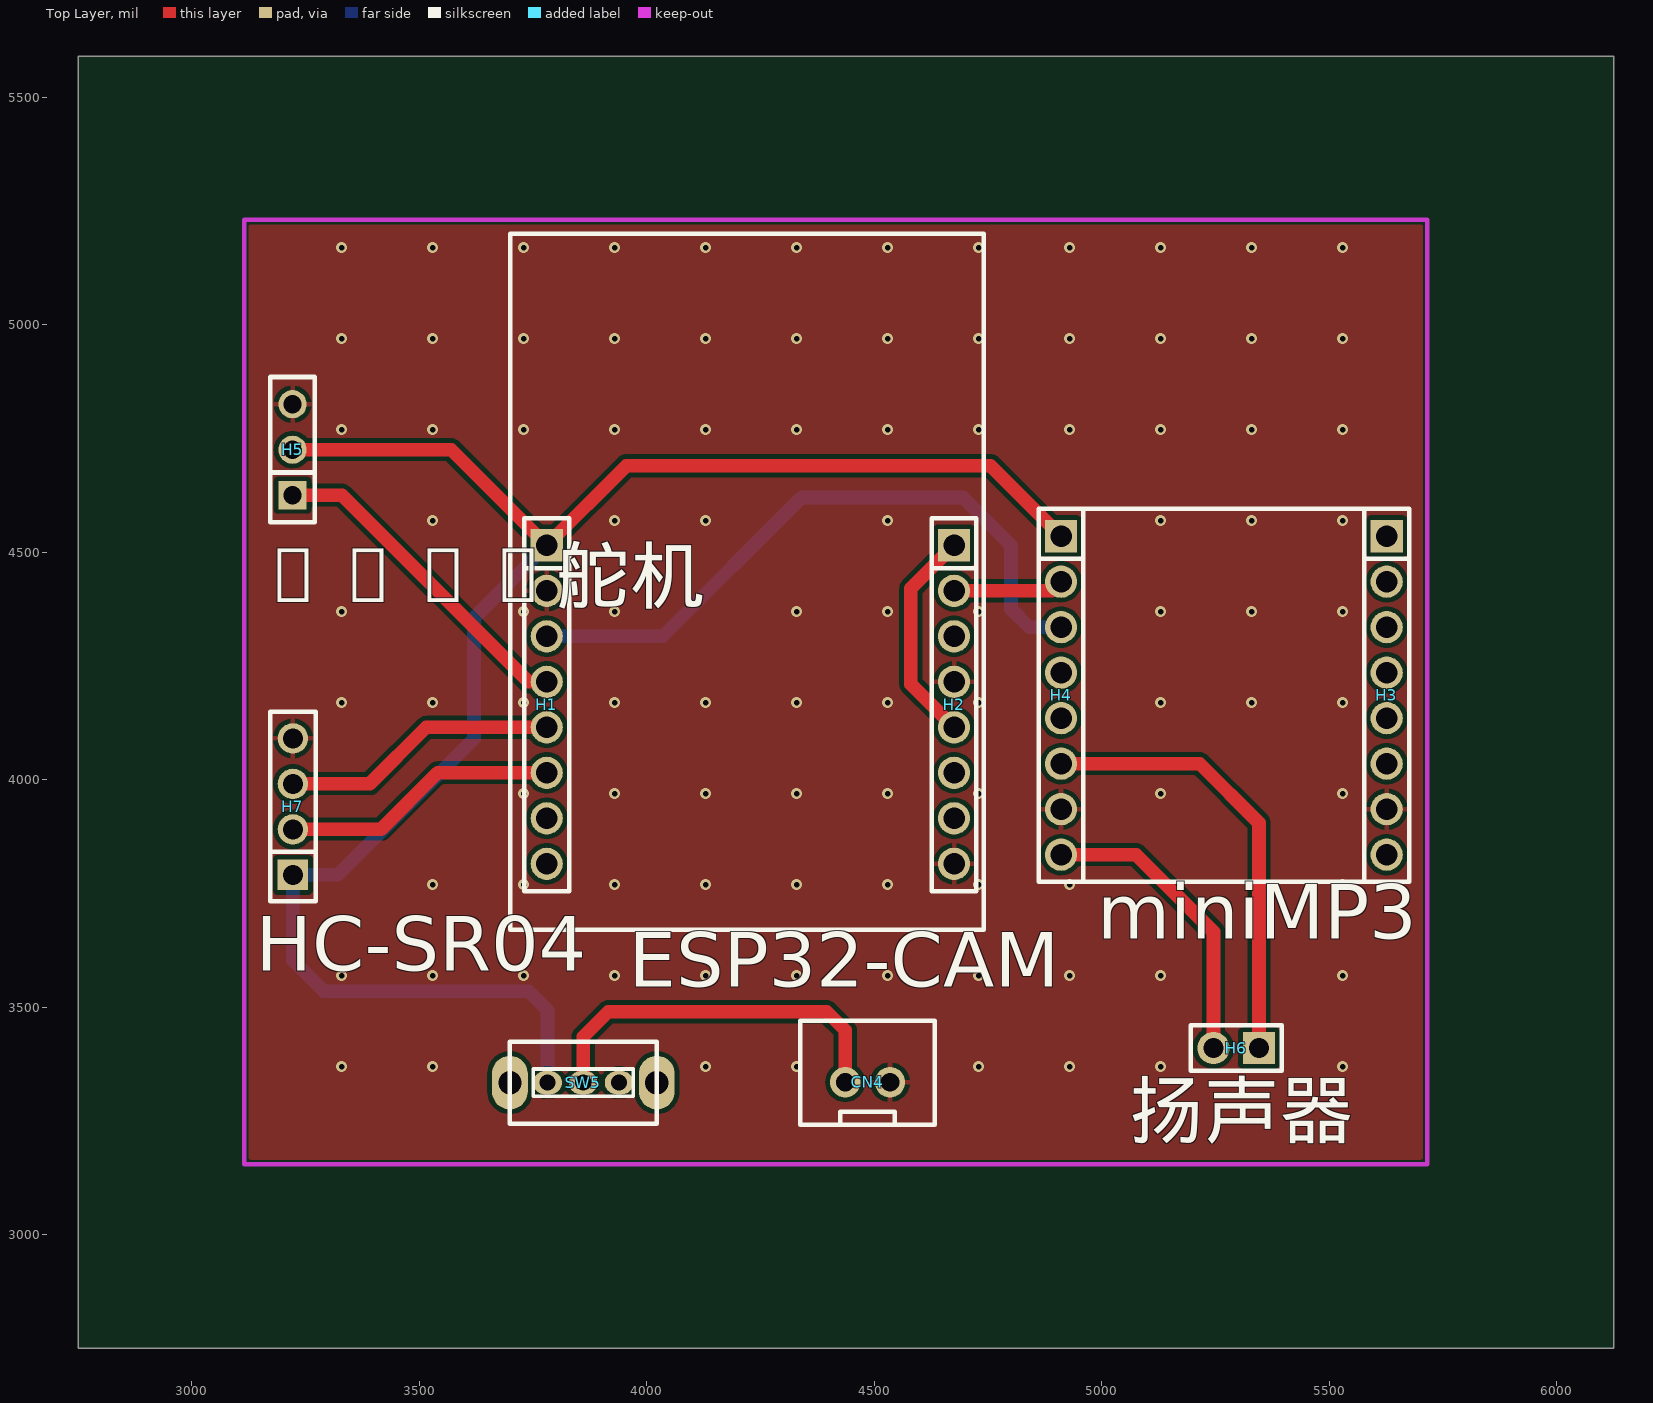
[diagram p0: Top Layer view]
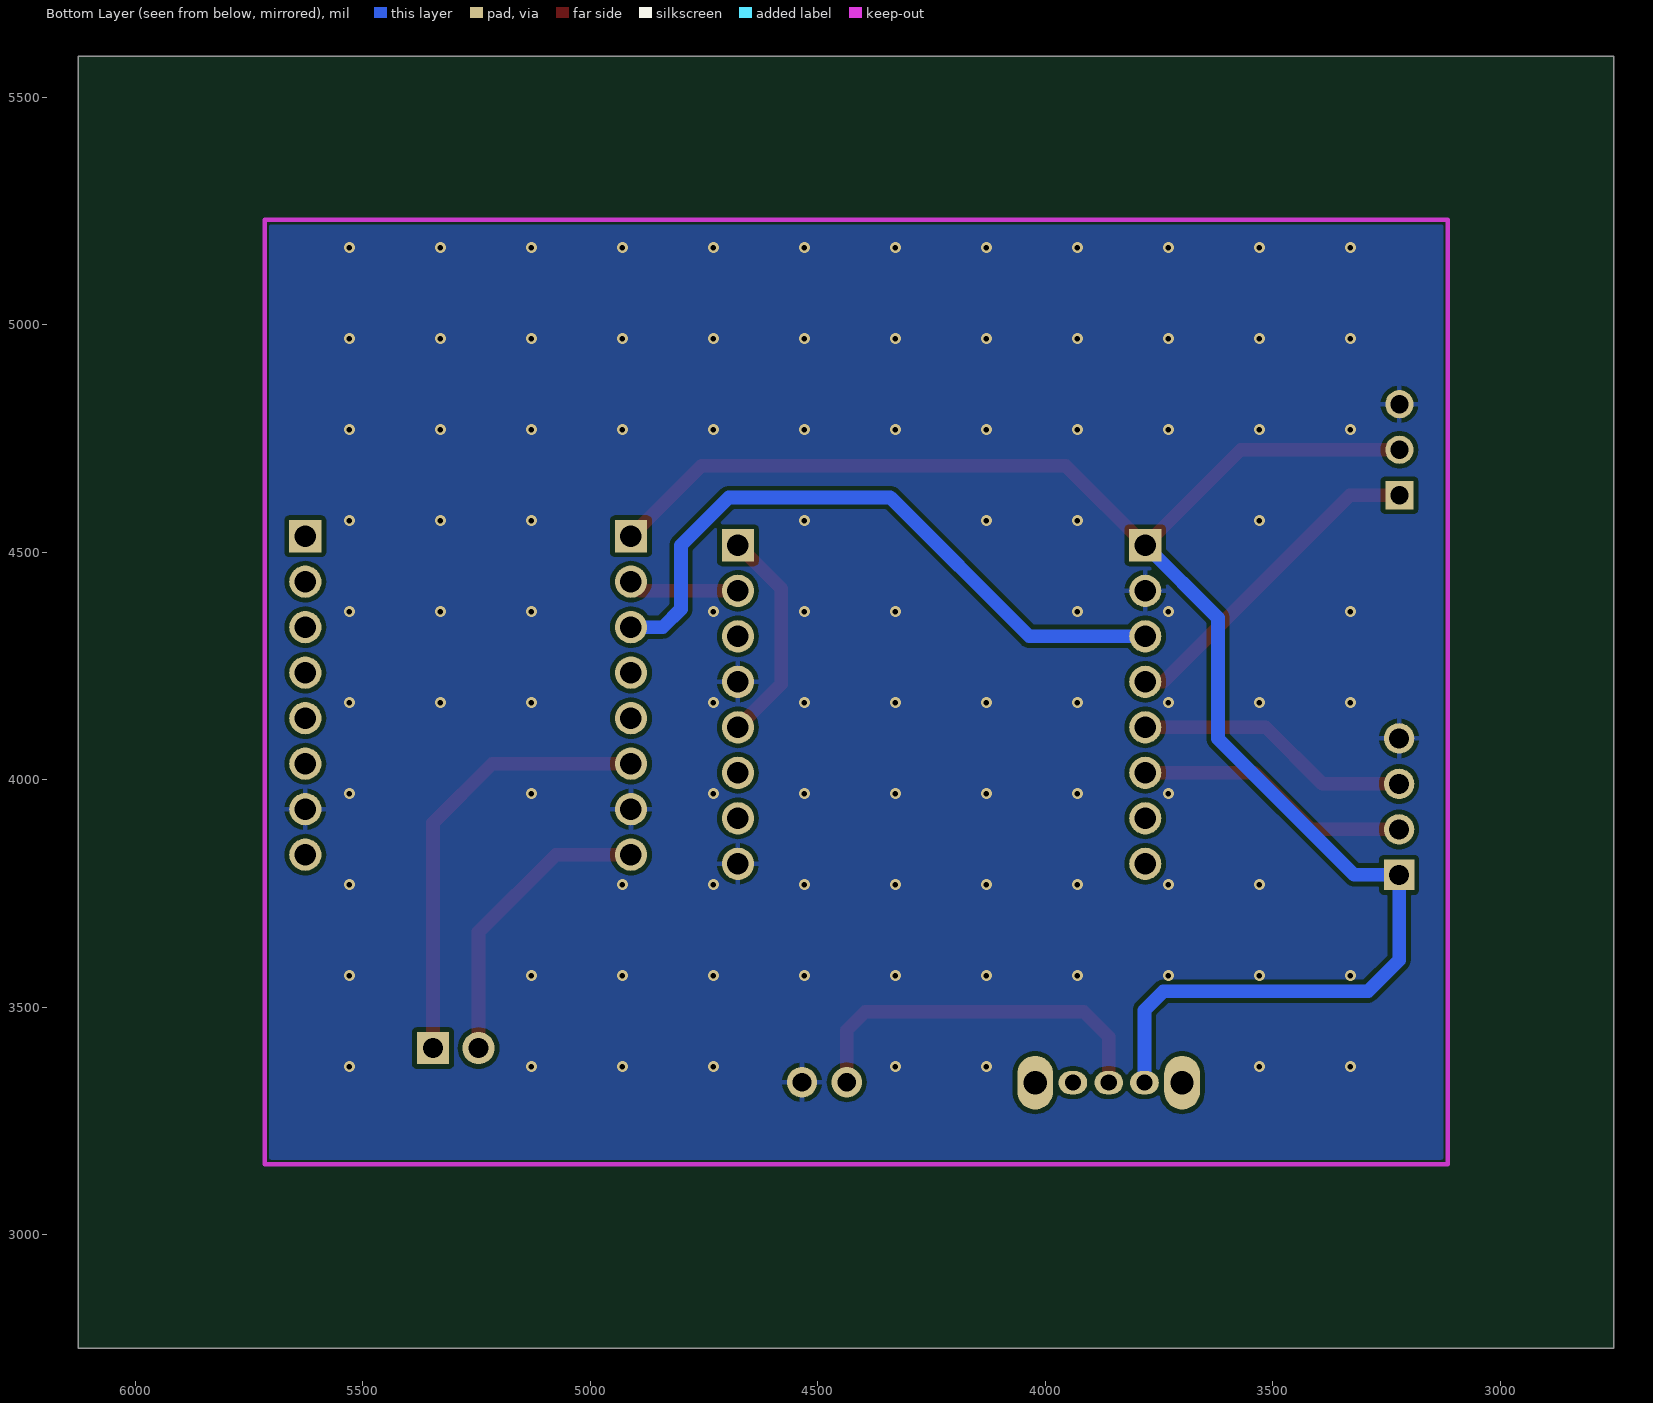
[diagram p1: Bottom Layer view, seen from below]
# Altium PCB MISC51682.pcbdoc
Units mil, origin at the board's own origin, x right, y up, seen from the top; angles counter-clockwise.
Board outline 3375 x 2840 mil, 2 copper layers (Top Layer, Bottom Layer), stack 62.206 mil thick; 9 components, 16 nets, 48 pads, 99 vias.

## Layer stack, top to bottom
Top Solder Mask Layer: solder mask 0.394, Dk 3.3
Top Layer: signal copper 1.379
Dielectric1: surface 59.449, FR4, Dk 4.5
Bottom Layer: signal copper 1.378
Bottom Solder Mask Layer: solder mask 0.394, Dk 3.3

## Board outline
6125,2750 2750,2750 2750,5590 6125,5590

## Design rules (kind name [scope] priority, off if disabled: settings)
BoardOutlineClearance copperThickness2oz_1 [All] p2 off: genericclearance=7.99 ignorepadtopadclearanceinfootprint=FALSE except(0: Arc-SplitContinuation Track-SplitContinuation SMDPad-SplitContinuation THPad-SplitContinuation Via-SplitContinuation Fill-SplitContinuation Region-SplitContinuation Poly-SplitContinuation Text-SplitContinuation Hole-SplitContinuation; 5.98: Arc-CutoutEdge Track-CutoutEdge SMDPad-CutoutEdge THPad-CutoutEdge Via-CutoutEdge Text-CutoutEdge; 6.9: Hole-OutlineEdge Hole-CutoutEdge; 10: Poly-OutlineEdge Poly-CutoutEdge; 11.81: Arc-OutlineEdge Track-OutlineEdge SMDPad-OutlineEdge THPad-OutlineEdge Via-OutlineEdge Fill-OutlineEdge Region-OutlineEdge Text-OutlineEdge Fill-CutoutEdge Region-CutoutEdge)
BoardOutlineClearance Plane_innerPlane_1 [All] p4 off: genericclearance=4.02 ignorepadtopadclearanceinfootprint=FALSE except(0: Arc-SplitContinuation Track-SplitContinuation SMDPad-SplitContinuation THPad-SplitContinuation Via-SplitContinuation Fill-SplitContinuation Region-SplitContinuation Poly-SplitContinuation Text-SplitContinuation Hole-SplitContinuation; 5.98: Arc-CutoutEdge Track-CutoutEdge SMDPad-CutoutEdge THPad-CutoutEdge Via-CutoutEdge Text-CutoutEdge; 6.9: Hole-OutlineEdge Hole-CutoutEdge; 10: Poly-OutlineEdge Poly-CutoutEdge; 11.81: Arc-OutlineEdge Track-OutlineEdge SMDPad-OutlineEdge THPad-OutlineEdge Via-OutlineEdge Fill-OutlineEdge Region-OutlineEdge Text-OutlineEdge Fill-CutoutEdge Region-CutoutEdge)
BoardOutlineClearance Copper_copperRegion_1 [All] p6 off: genericclearance=4.02 ignorepadtopadclearanceinfootprint=FALSE except(0: Arc-SplitContinuation Track-SplitContinuation SMDPad-SplitContinuation THPad-SplitContinuation Via-SplitContinuation Fill-SplitContinuation Region-SplitContinuation Poly-SplitContinuation Text-SplitContinuation Hole-SplitContinuation; 5.98: Arc-CutoutEdge Track-CutoutEdge SMDPad-CutoutEdge THPad-CutoutEdge Via-CutoutEdge Text-CutoutEdge; 6.9: Hole-OutlineEdge Hole-CutoutEdge; 10: Poly-OutlineEdge Poly-CutoutEdge; 11.81: Arc-OutlineEdge Track-OutlineEdge SMDPad-OutlineEdge THPad-OutlineEdge Via-OutlineEdge Fill-OutlineEdge Region-OutlineEdge Text-OutlineEdge Fill-CutoutEdge Region-CutoutEdge)
BoardOutlineClearance copperThickness1oz_1 [All] p8: genericclearance=4.02 ignorepadtopadclearanceinfootprint=FALSE except(0: Arc-SplitContinuation Track-SplitContinuation SMDPad-SplitContinuation THPad-SplitContinuation Via-SplitContinuation Fill-SplitContinuation Region-SplitContinuation Poly-SplitContinuation Text-SplitContinuation Hole-SplitContinuation; 5.98: Arc-CutoutEdge Track-CutoutEdge SMDPad-CutoutEdge THPad-CutoutEdge Via-CutoutEdge Text-CutoutEdge; 6.9: Hole-OutlineEdge Hole-CutoutEdge; 10: Poly-OutlineEdge Poly-CutoutEdge; 11.81: Arc-OutlineEdge Track-OutlineEdge SMDPad-OutlineEdge THPad-OutlineEdge Via-OutlineEdge Fill-OutlineEdge Region-OutlineEdge Text-OutlineEdge Fill-CutoutEdge Region-CutoutEdge)
Clearance copperThickness2oz [All] p1 off: gap=7.99 ignorepadtopadclearanceinfootprint=FALSE except(5.98: SMDPad-Track SMDPad-SMDPad THPad-Track SMDPad-THPad THPad-THPad Track-Via SMDPad-Via THPad-Via Via-Via Fill-SMDPad Region-SMDPad Fill-THPad Region-THPad Fill-Via Region-Via Fill-Fill Fill-Region Region-Region Arc-Track Arc-SMDPad Arc-THPad Arc-Via Fill-Arc Region-Arc Arc-Arc Text-Track SMDPad-Text Text-THPad Text-Via Fill-Text Region-Text Arc-Text Text-Text; 6.9: Hole-Track Hole-SMDPad Hole-THPad Hole-Via Fill-Hole Region-Hole Hole-Arc Hole-Text; 10: Poly-Track Poly-SMDPad Poly-THPad Poly-Via Poly-Fill Poly-Region Poly-Poly Poly-Arc Poly-Text Poly-Hole; 11.81: Fill-Track Region-Track)
Clearance Plane_innerPlane [All] p3 off: gap=4.02 ignorepadtopadclearanceinfootprint=FALSE except(5.98: SMDPad-Track SMDPad-SMDPad THPad-Track SMDPad-THPad THPad-THPad Track-Via SMDPad-Via THPad-Via Via-Via Fill-SMDPad Region-SMDPad Fill-THPad Region-THPad Fill-Via Region-Via Fill-Fill Fill-Region Region-Region Arc-Track Arc-SMDPad Arc-THPad Arc-Via Fill-Arc Region-Arc Arc-Arc Text-Track SMDPad-Text Text-THPad Text-Via Fill-Text Region-Text Arc-Text Text-Text; 6.9: Hole-Track Hole-SMDPad Hole-THPad Hole-Via Fill-Hole Region-Hole Hole-Arc Hole-Text; 10: Poly-Track Poly-SMDPad Poly-THPad Poly-Via Poly-Fill Poly-Region Poly-Poly Poly-Arc Poly-Text Poly-Hole; 11.81: Fill-Track Region-Track)
Clearance Copper_copperRegion [All] p5 off: gap=4.02 ignorepadtopadclearanceinfootprint=FALSE except(5.98: SMDPad-Track SMDPad-SMDPad THPad-Track SMDPad-THPad THPad-THPad Track-Via SMDPad-Via THPad-Via Via-Via Fill-SMDPad Region-SMDPad Fill-THPad Region-THPad Fill-Via Region-Via Fill-Fill Fill-Region Region-Region Arc-Track Arc-SMDPad Arc-THPad Arc-Via Fill-Arc Region-Arc Arc-Arc Text-Track SMDPad-Text Text-THPad Text-Via Fill-Text Region-Text Arc-Text Text-Text; 6.9: Hole-Track Hole-SMDPad Hole-THPad Hole-Via Fill-Hole Region-Hole Hole-Arc Hole-Text; 10: Poly-Track Poly-SMDPad Poly-THPad Poly-Via Poly-Fill Poly-Region Poly-Poly Poly-Arc Poly-Text Poly-Hole; 11.81: Fill-Track Region-Track)
Clearance copperThickness1oz [All] p7: gap=4.02 ignorepadtopadclearanceinfootprint=FALSE except(5.98: SMDPad-Track SMDPad-SMDPad THPad-Track SMDPad-THPad THPad-THPad Track-Via SMDPad-Via THPad-Via Via-Via Fill-SMDPad Region-SMDPad Fill-THPad Region-THPad Fill-Via Region-Via Fill-Fill Fill-Region Region-Region Arc-Track Arc-SMDPad Arc-THPad Arc-Via Fill-Arc Region-Arc Arc-Arc Text-Track SMDPad-Text Text-THPad Text-Via Fill-Text Region-Text Arc-Text Text-Text; 6.9: Hole-Track Hole-SMDPad Hole-THPad Hole-Via Fill-Hole Region-Hole Hole-Arc Hole-Text; 10: Poly-Track Poly-SMDPad Poly-THPad Poly-Via Poly-Fill Poly-Region Poly-Poly Poly-Arc Poly-Text Poly-Hole; 11.81: Fill-Track Region-Track)
DiffPairsRouting differentialPair [All] p1: maxlimit=6 minlimit=6 mostfreqgap=6 toplayer_minwidth=5 toplayer_prefwidth=10 toplayer_maxwidth=100 toplayer_mingap=6 toplayer_prefgap=6 toplayer_maxgap=6 bottomlayer_minwidth=5 bottomlayer_prefwidth=10 bottomlayer_maxwidth=100 bottomlayer_mingap=6 bottomlayer_prefgap=6 bottomlayer_maxgap=6 maxuncoupledlength=10
HoleToHoleClearance otherClearance [All] p1: gap=11.81 allowstackedmicrovias=TRUE
Length netLength [All] p1: minlimit=0 maxlimit=0
PasteMaskExpansion pasteMaskExpansion [All] p1: expansion=0
PlaneConnect innerPlane [All] p1: planeconnectstyle=Relief reliefexpansion=20 reliefentries=4 reliefconductorwidth=10 reliefairgap=10
PolygonConnect copperRegion [(InNet('GND'))] p1: connectstyle=Relief reliefconductorwidth=10 reliefentries=4 polygonreliefangle="90 Angle" airgapwidth=10 via.connectstyle=Relief via.reliefconductorwidth=10 via.reliefentries=4 via.polygonreliefangle="90 Angle" via.airgapwidth=10
RoutingVias viaSize [All] p1: holewidth=12.01 width=24.02 viastyle="Through Hole" minholewidth=11.81 minwidth=19.68 maxholewidth=248.03 maxwidth=393.7
SolderMaskExpansion solderMaskExpansion [IsVia] p1: expansion=-1000 istentingtop=TRUE
SolderMaskExpansion solderMaskExpansion [All] p2: expansion=2 istentingtop=FALSE
Width copperThickness2oz_2 [All] p1 off: maxlimit=100 minlimit=8 preferedwidth=10
Width copperThickness1oz_2 [All] p2: maxlimit=100 minlimit=5 preferedwidth=10

## Components (designator, comment, footprint, x,y, rotation, side; value= is the part's Value field where it differs from the comment)
CN4 "XH2.54*2P_直插" CONN-TH_2P-P2.50-XH2.54-2P 4485,3335 r180 top
H1 "" HDR-TH_8P-P2.54-V-F-1 3779.84,4165 r270 top
H2 "" HDR-TH_8P-P2.54-V-F-1 4675,4165 r270 top
H3 "" HDR-TH_8P-P2.54-V-F-1 5625.77,4185 r270 top
H4 "" HDR-TH_8P-P2.54-V-F-1 4910,4185 r270 top
H5 "" HDR-TH_3P-P2.54-V-F 3221.22,4725 r90 top
H6 "" HDR-TH_2P-P2.54-V-M-1 5295,3410 r180 top
H7 "" HDR-TH_4P-P2.54-V-F 3222.01,3940.62 r90 top
SW5 "" 拨动开关 3855,3334 r0 top

## Footprints (in the part's own frame and the unit in brackets; to place one, negate y for a bottom-side part, rotate by r counter-clockwise, add the part's x,y. Pads: shape width x height; smd on the part's side, far side on the other; paste and mask are expansions set on the pad)
CONN-TH_2P-P2.50-XH2.54-2P [mm]
  round 1.7 hole 1.05 paste+0 mask+0.05: 1(1.25,0) 2(-1.25,0)
  silkscreen extent -3.75,-3.42 3.75,2.37
HDR-TH_2P-P2.54-V-M-1 [mm]
  rect 1.8x1.8 hole 1.1: 1(-1.27,0)
  round 1.8 hole 1.1: 2(1.27,0)
  silkscreen extent -2.54,-1.27 2.54,1.27
HDR-TH_3P-P2.54-V-F [mil]
  rect 62x62 hole 40.16: 1(-100,0)
  round 62 hole 40.16: 2(0,0) 3(100,0)
  silkscreen extent -160,-49 160,49
HDR-TH_4P-P2.54-V-F [mm]
  rect 1.7x1.7 hole 1.1: 1(-3.81,0)
  round 1.7 hole 1.1: 2(-1.27,0) 3(1.27,0) 4(3.81,0)
  silkscreen extent -5.29,-1.27 5.29,1.27
HDR-TH_8P-P2.54-V-F-1 [mm]
  rect 1.8x1.8 hole 1.2: 1(-8.89,0)
  round 1.8 hole 1.2: 2(-6.35,0) 3(-3.81,0) 4(-1.27,0) 5(1.27,0) 6(3.81,0) 7(6.35,0) 8(8.89,0)
  silkscreen extent -10.41,-1.25 10.41,1.25
拨动开关 [mil]
  oval 63x51.2 hole 35.4 paste+0 mask+2: 1(-73.4,0) 2(5,0) 3(84,0)
  oval 78.7x118.1 hole 51.2 paste+0 mask+2: 4(166.7,0) 5(-156.1,0)
  silkscreen extent -156,-90 167,90

## Via types
v1: diameter 24.02, hole 12, Top Layer to Bottom Layer, 99 vias

## Nets (pads, with @x,y where several pads share a name; then routed paths per layer and width w, separated by ;. In a path a pad name is that pad's centre, name@x,y a point inside that pad or via, vN(x,y) a via of type N, cw(c..) or ccw(c..) an arc to the next point about the centre after c; other vN are vias at no path point)
$1N17118: CN4.1 SW5.2 | length 830.7
  Top Layer w30: SW5.2 3860,3435 3915,3490 4395,3490 4435.78,3449.22 CN4.1
$1N17161: H4.6 H6.1 | length 983.8
  Top Layer w30: H4.6 5215,4035 5345,3905 H6.1
$1N17162: H4.8 H6.2 | length 660.4
  Top Layer w30: H4.8 5075,3835 5245,3665 H6.2
+5V: H1.1 H4.1 H5.2 H7.1 SW5.1 | length 3877.7
  Top Layer w30: H5.2 3569.84,4725 H1.1 3954.84,4690 4755,4690 H4.1
  Bottom Layer w30: H1.1 3620,4355.16 3620,4090 3320.62,3790.62 H7.1 3222.01,3602.99 3290,3535 3740,3535 3781.6,3493.4 SW5.1
GND: CN4.2 H1.2 H2.4 H2.8 H3.7 H4.7 H5.3 H7.4
  other v1: 3329.1,3369.1 3529.1,3369.1 4129.1,3369.1 4329.1,3369.1 4729.1,3369.1 4929.1,3369.1 5129.1,3369.1 5529.1,3369.1 3329.1,3569.1 3529.1,3569.1 3729.1,3569.1 3929.1,3569.1 4129.1,3569.1 4329.1,3569.1 4529.1,3569.1 4729.1,3569.1 4929.1,3569.1 5129.1,3569.1 5529.1,3569.1 3529.1,3769.1 3729.1,3769.1 3929.1,3769.1 4129.1,3769.1 4329.1,3769.1 4529.1,3769.1 4729.1,3769.1 4929.1,3769.1 5529.1,3769.1 3729.1,3969.1 3929.1,3969.1 4129.1,3969.1 4329.1,3969.1 4529.1,3969.1 4729.1,3969.1 5129.1,3969.1 5529.1,3969.1 3329.1,4169.1 3529.1,4169.1 3729.1,4169.1 3929.1,4169.1 4129.1,4169.1 4329.1,4169.1 4529.1,4169.1 4729.1,4169.1 5129.1,4169.1 5329.1,4169.1 5529.1,4169.1 3329.1,4369.1 3729.1,4369.1 3929.1,4369.1 4329.1,4369.1 4529.1,4369.1 4729.1,4369.1 5129.1,4369.1 5329.1,4369.1 5529.1,4369.1 3529.1,4569.1 3929.1,4569.1 4129.1,4569.1 4529.1,4569.1 5129.1,4569.1 5329.1,4569.1 5529.1,4569.1 3329.1,4769.1 3529.1,4769.1 3729.1,4769.1 3929.1,4769.1 4129.1,4769.1 4329.1,4769.1 4529.1,4769.1 4729.1,4769.1 4929.1,4769.1 5129.1,4769.1 5329.1,4769.1 5529.1,4769.1 3329.1,4969.1 3529.1,4969.1 3729.1,4969.1 3929.1,4969.1 4129.1,4969.1 4329.1,4969.1 4529.1,4969.1 4729.1,4969.1 4929.1,4969.1 5129.1,4969.1 5329.1,4969.1 5529.1,4969.1 3329.1,5169.1 3529.1,5169.1 3729.1,5169.1 3929.1,5169.1 4129.1,5169.1 4329.1,5169.1 4529.1,5169.1 4729.1,5169.1 4929.1,5169.1 5129.1,5169.1 5329.1,5169.1 5529.1,5169.1
IO0: H2.3
IO2: H1.7
IO4: H1.8
IO12: H1.3 H4.3 | length 1456.6
  Bottom Layer w30: H1.3 4035,4315 4340,4620 4695,4620 4800,4515 4800,4375 4840,4335 H4.3
IO13: H1.4 H5.1 | length 728.5
  Top Layer w30: H5.1 3330,4625 3740,4215 H1.4
IO14: H1.6 H7.2 | length 609.4
  Top Layer w30: H7.2 3415.62,3890.62 3540,4015 H1.6
IO15: H1.5 H7.3 | length 609.4
  Top Layer w30: H7.3 3390.62,3990.62 3515,4115 H1.5
IO16: H2.2 H4.2 | length 243.3
  Top Layer w30: H2.2 4890,4415 H4.2
VCC: H2.1 H2.5 | length 478.7
  Top Layer w30: H2.5 4580,4210 4580,4420 H2.1
VDT: H2.7
VOR: H2.6
pads on no net: H3.1 H3.2 H3.3 H3.4 H3.5 H3.6 H3.8 H4.4 H4.5 SW5.3 SW5.4 SW5.5

## Polygon pours and split planes (outlines as drawn)
GND on Bottom Layer (solid, remove dead copper, pour order 2): 3000,5325 3000,3000 5835,3000 5835,5325
GND on Top Layer (solid, remove dead copper, pour order 0): 3060,5340 3060,3045 5875,3045 5875,5340

## Keep-outs
Board Outline Layer:
  lines w10: 3115,3155 3115,5230 5715,5230 5715,3155 3115,3155

## Silkscreen, mask and mechanical layers (free items; w line width, h text height)
Top Silkscreen Layer:
  lines w10: 3700,3670 3700,5200 4740,5200 4740,3670 3700,3670 ; 4860.79,3775.16 4860.79,4594.84 5674.98,4594.84 5674.98,3775.16 4860.79,3775.16
  text "SG90舵机" at 3140,4390 h120
  text "miniMP3" at 4990,3650 h120
  text "HC-SR04" at 3140,3580 h120
  text "ESP32-CAM" at 3960,3545 h120
  text "扬声器" at 5060,3215 h120